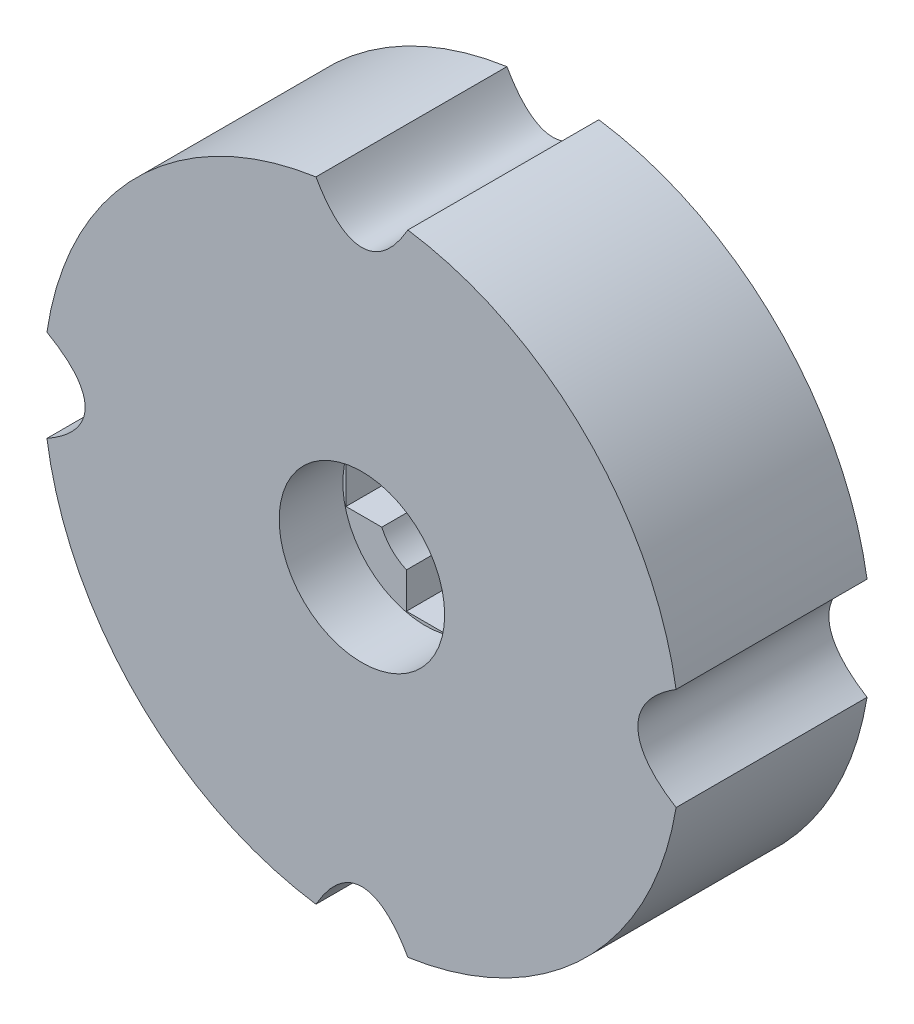
from build123d import *

# Parameters (mm, degrees)
EXTRUDE_1_DEPTH     = 15
SKETCH_2_R          = 13
CUT_EXTRUDE_2_DEPTH = 10


with BuildPart() as part:
    # 草图1 → 拉伸1 (new, symmetric)
    with BuildSketch(Plane.XY):
        with BuildLine():
            ThreePointArc((-7.220859013, 49.475844562), (-35.355230678, 35.355447441), (-49.47580029, 7.221162349))
            add(Edge.make_bspline(
                [(-49.47580029, -7.221162349), (-36.725591286, 0), (-49.47580029, 7.221162349)],
                knots=[2.665650331, 2.665650331, 2.665650331, 3.617534976, 3.617534976, 3.617534976], degree=2, weights=[1, 0.888861367, 1]))
            ThreePointArc((-49.47580029, -7.221162349), (-35.355230678, -35.355447441), (-7.220859013, -49.475844562))
            add(Edge.make_bspline(
                [(7.220859013, -49.475844562), (0, -36.72563521), (-7.220859013, -49.475844562)],
                knots=[2.665650231, 2.665650231, 2.665650231, 3.617535076, 3.617535076, 3.617535076], degree=2, weights=[1, 0.888861321, 1]))
            ThreePointArc((7.220859013, -49.475844562), (35.063945901, -35.644350154), (49.350641932, -8.032069525))
            add(Edge.make_bspline(
                [(49.350641932, 8.032069525), (36.37710154, 0), (49.350641932, -8.032069525)],
                knots=[5.748433423, 5.748433423, 5.748433423, 6.817937192, 6.817937192, 6.817937192], degree=2, weights=[1, 0.860395102, 1]))
            ThreePointArc((49.350641932, 8.032069525), (35.063945901, 35.644350154), (7.220859013, 49.475844562))
            add(Edge.make_bspline(
                [(-7.220859013, 49.475844562), (0, 36.72563521), (7.220859013, 49.475844562)],
                knots=[2.665650231, 2.665650231, 2.665650231, 3.617535076, 3.617535076, 3.617535076], degree=2, weights=[1, 0.888861321, 1]))
        make_face()
        with BuildLine():
            Line((3, -6.873863542), (3, -12.5))
            Line((3, -12.5), (-3, -12.5))
            Line((-3, -12.5), (-3, -6.873863542))
            ThreePointArc((-3, -6.873863542), (-5.303300859, -5.303300859), (-6.873863542, -3))
            Line((-6.873863542, -3), (-12.5, -3))
            Line((-12.5, -3), (-12.5, 3))
            Line((-12.5, 3), (-6.873863542, 3))
            ThreePointArc((-6.873863542, 3), (-5.303300859, 5.303300859), (-3, 6.873863542))
            Line((-3, 6.873863542), (-3, 12.5))
            Line((-3, 12.5), (3, 12.5))
            Line((3, 12.5), (3, 6.873863542))
            ThreePointArc((3, 6.873863542), (5.303300859, 5.303300859), (6.873863542, 3))
            Line((6.873863542, 3), (12.5, 3))
            Line((12.5, 3), (12.5, -3))
            Line((12.5, -3), (6.873863542, -3))
            ThreePointArc((6.873863542, -3), (5.303300859, -5.303300859), (3, -6.873863542))
        make_face(mode=Mode.SUBTRACT)
    extrude(amount=EXTRUDE_1_DEPTH, both=True)

    # 草图2 → 拉伸2 (cut)
    with BuildSketch(Plane.XY.offset(15)):
        Circle(SKETCH_2_R)
    extrude(amount=-CUT_EXTRUDE_2_DEPTH, mode=Mode.SUBTRACT)


solid = part.part
